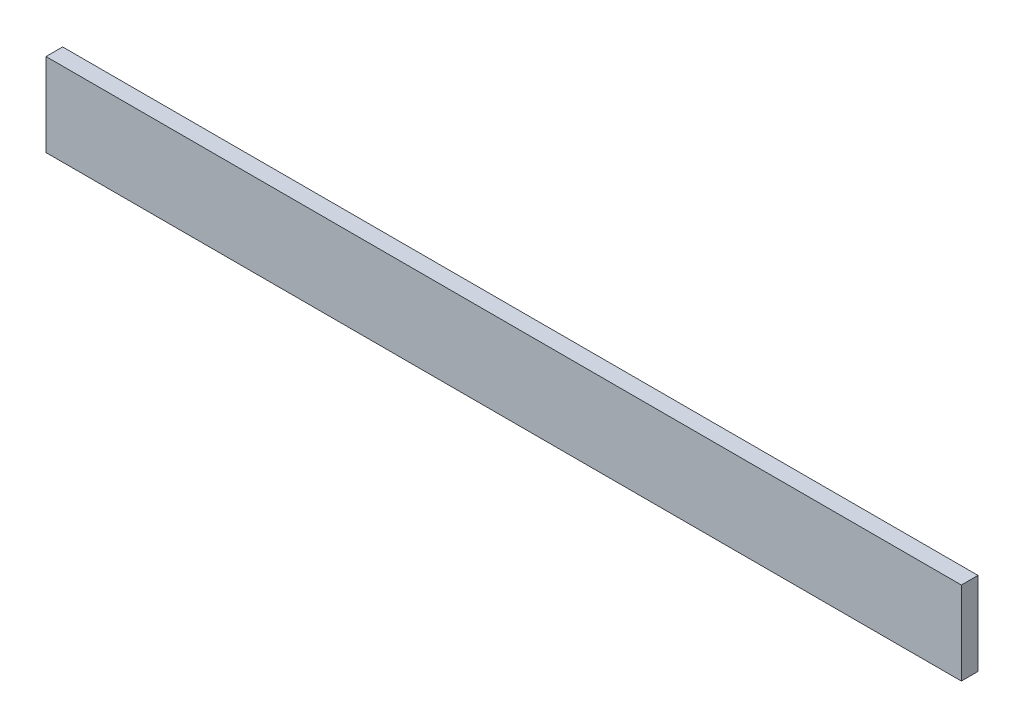
from build123d import *

# Parameters (mm, degrees)
SKETCH1_W           = 1100
SKETCH1_H           = 100
BOSS_EXTRUDE1_DEPTH = 20


with BuildPart() as part:
    # Sketch1 → Boss-Extrude1 (new body)
    with BuildSketch(Plane.XY):
        with Locations((550, 50)):
            Rectangle(SKETCH1_W, SKETCH1_H)
    extrude(amount=BOSS_EXTRUDE1_DEPTH)


solid = part.part
